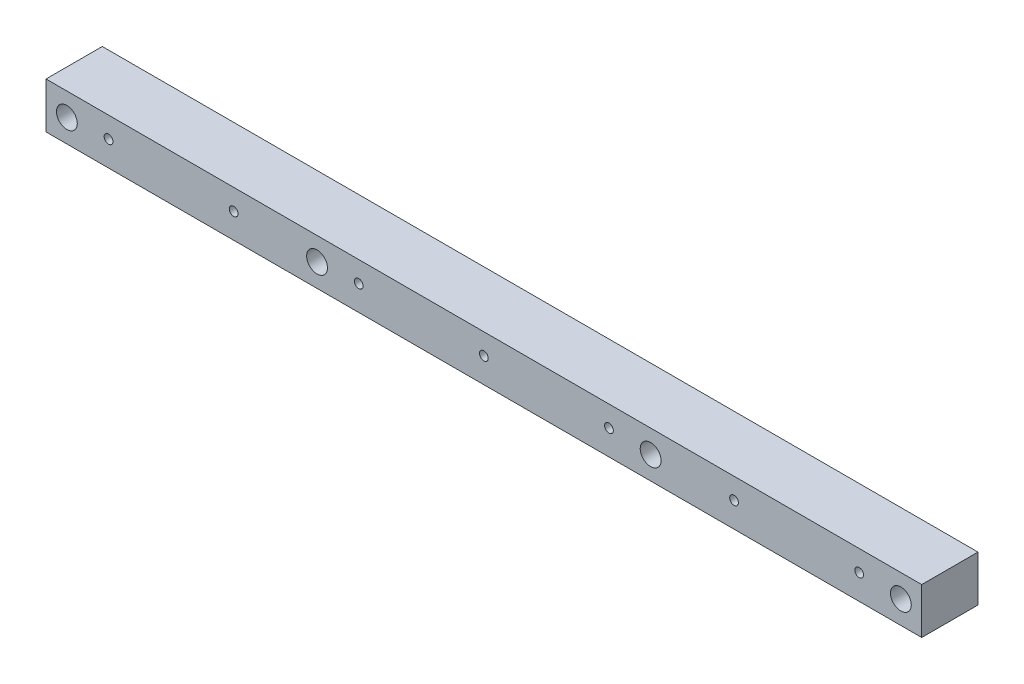
SolidWorks part; units mm, degrees
ref_plane "Front Plane" through (0, 0, 0) normal (0, 0, 1) x (1, 0, 0)
ref_plane "Top Plane" through (0, 0, 0) normal (0, 1, 0) x (1, 0, 0)
ref_plane "Right Plane" through (0, 0, 0) normal (1, 0, 0) x (0, 0, -1)
sketch "Sketch1" plane through (0, 0, 0) normal (0, 0, 1) x (1, 0, 0)
  line L1 (-210, -11) -> (210, -11)
  line L2 (-210, -11) -> (-210, 11)
  line L3 (-210, 11) -> (210, 11)
  line L4 (210, -11) -> (210, 11)
  line L5 (-210, -11) -> (210, 11) construction
  line L6 (-210, 11) -> (210, -11) construction
  point P0 (0, 0)
  dimension "D1" = 420
  dimension "D2" = 22
extrude "Boss-Extrude1" add sketch "Sketch1" along normal blind 27
hole_wizard "M5 Tapped Hole1" positions "Sketch2" profile "Sketch3" tap size "M5" standard "ISO"
sketch "Sketch2" plane through (0, 0, 27) normal (0, 0, 1) x (1, 0, 0)
  point P0 (-180, 1)
  point P3 (-120, 1)
  point P6 (-60, 1)
  point P9 (0, 1)
  point P12 (60, 1)
  point P15 (120, 1)
  point P18 (180, 1)
sketch "Sketch3" plane through (-180, 1, 27) normal (1, 0, 0) x (0, -1, 0)
  line L0 (0, 0) -> (0, 13.6618)
  line L1 (0, 13.6618) -> (2.1, 12.4)
  line L2 (2.1, 12.4) -> (2.1, 0)
  line L5 (2.1, 0) -> (0, 0)
  line L10 (0, 13.6618) -> (-2.1, 12.4) construction
  line L11 (0, -6.35) -> (0, 107.95) construction
  dimension "螺纹孔钻头直径" = 4.2
  dimension "螺纹孔钻头深度" = 12.4
  dimension "导头角度" = 118
cosmetic thread "Cosmetic Thread1"
cosmetic thread "Cosmetic Thread2"
cosmetic thread "Cosmetic Thread3"
cosmetic thread "Cosmetic Thread4"
cosmetic thread "Cosmetic Thread5"
cosmetic thread "Cosmetic Thread6"
cosmetic thread "Cosmetic Thread7"
hole_wizard "CBORE for M5 Hex Socket Head Cap Screw1" positions "Sketch4" profile "Sketch5" counterbore size "M5" standard "ISO" end condition through all
sketch "Sketch4" plane through (0, 0, 27) normal (0, 0, 1) x (1, 0, 0)
  line L0 (-200, 0) -> (-80, 0) construction
  line L1 (-80, 0) -> (0, 0) construction
  line L2 (0, 0) -> (0, 77.6318) construction
  line L3 (200, 0) -> (80, 0) construction
  point P0 (-200, 0)
  point P2 (-80, 0)
  point P17 (80, 0)
  point P20 (200, 0)
  dimension "D1" = 160
  dimension "D2" = 120
sketch "Sketch5" plane through (-200, 0, 27) normal (1, 0, 0) x (0, -1, 0)
  line L0 (0, 0) -> (0, 27)
  line L1 (0, 27) -> (2.75, 27)
  line L3 (2.75, 27) -> (2.75, 17)
  line L4 (2.75, 17) -> (5, 17)
  line L5 (5, 17) -> (5, 0)
  line L7 (5, 0) -> (0, 0)
  line L11 (0, -6.35) -> (0, 107.95) construction
  dimension "通孔孔直径" = 5.5
  dimension "通孔孔深度" = 27
  dimension "柱形沉头孔直径" = 10
  dimension "柱形沉头孔深度" = 17
